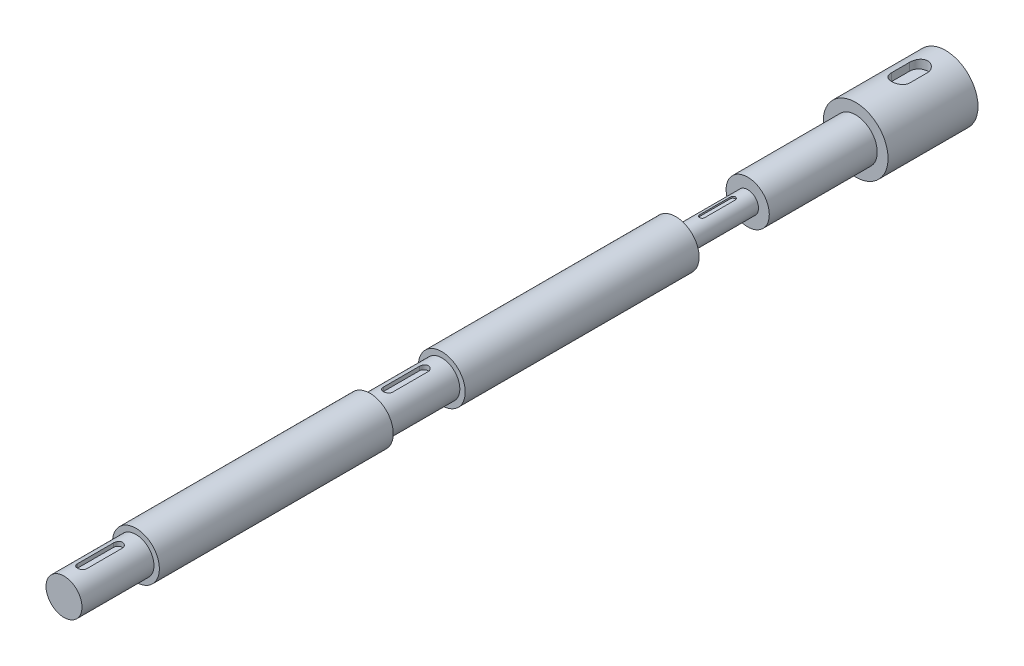
from build123d import *
from build123d.topology import SkipClean

# Parameters (mm, degrees)
SKETCH1_R           = 18
BOSS_EXTRUDE2_DEPTH = 25
SKETCH6_R           = 12
BOSS_EXTRUDE6_DEPTH = 60
SKETCH7_R           = 6
BOSS_EXTRUDE7_DEPTH = 30
CUT_EXTRUDE3_DEPTH  = 10
CUT_EXTRUDE4_DEPTH  = 5
CUT_EXTRUDE5_DEPTH  = 2.5
CUT_EXTRUDE6_DEPTH  = 2.5


with BuildPart() as part:
    # Sketch1 → Boss-Extrude2 (new, symmetric)
    with BuildSketch(Plane.XY):
        Circle(SKETCH1_R)
    extrude(amount=BOSS_EXTRUDE2_DEPTH, both=True)

    # Sketch6 → Boss-Extrude6 (add)
    with BuildSketch(Plane.XY.offset(25)):
        Circle(SKETCH6_R)
    extrude(amount=BOSS_EXTRUDE6_DEPTH)

    # Sketch7 → Boss-Extrude7 (add)
    with BuildSketch(Plane.XY.offset(85)):
        Circle(SKETCH7_R)
    extrude(amount=BOSS_EXTRUDE7_DEPTH)

    # Sketch11 → Cut-Extrude3 (cut)
    with BuildSketch(Plane(origin=(0, 13, 0), x_dir=(-1, 0, 0), z_dir=(0, 1, 0))):
        with BuildLine():
            Line((-5, 0), (-5, -10))
            ThreePointArc((-5, -10), (0, -15), (5, -10))
            Line((5, -10), (5, 0))
            ThreePointArc((5, 0), (0, 5), (-5, 0))
        make_face()
    extrude(amount=CUT_EXTRUDE3_DEPTH, mode=Mode.SUBTRACT)

    # Sketch12 → Cut-Extrude4 (cut)
    with BuildSketch(Plane(origin=(0, 5, 0), x_dir=(-1, 0, 0), z_dir=(0, 1, 0))):
        with BuildLine():
            Line((-1.4, 110.5), (-1.4, 93.3))
            ThreePointArc((-1.4, 93.3), (0, 91.9), (1.4, 93.3))
            Line((1.4, 93.3), (1.4, 110.5))
            ThreePointArc((1.4, 110.5), (0, 111.9), (-1.4, 110.5))
        make_face()
    extrude(amount=CUT_EXTRUDE4_DEPTH, mode=Mode.SUBTRACT)

    # Sketch13 → Revolve1 (revolve)
    with SkipClean():  # the faces are left unmerged after this step: merging them gives an invalid solid
        with BuildSketch(Plane(origin=(0, 0, 0), x_dir=(1, 0, 0), z_dir=(0, 1, 0))):
            Polygon((0, -465), (0, -115), (-6, -115), (-6, -125), (-13, -125), (-13, -255), (-10, -255), (-10, -295), (-13, -295), (-13, -425), (-10, -425), (-10, -465), align=None)
        revolve(axis=Axis((0, 0, 75.161405529), (0, 0, 1)))

    # Sketch16 → Cut-Extrude5 (cut)
    with SkipClean():  # the faces are left unmerged after this step: merging them gives an invalid solid
        with BuildSketch(Plane(origin=(0, 10, 0), x_dir=(1, 0, 0), z_dir=(0, 1, 0))):
            with BuildLine():
                Line((2.5, -265), (2.5, -285))
                ThreePointArc((2.5, -285), (0, -287.5), (-2.5, -285))
                Line((-2.5, -285), (-2.5, -265))
                ThreePointArc((-2.5, -265), (0, -262.5), (2.5, -265))
            make_face()
        extrude(amount=-CUT_EXTRUDE5_DEPTH, mode=Mode.SUBTRACT)

    # Sketch17 → Cut-Extrude6 (cut)
    with SkipClean():  # the faces are left unmerged after this step: merging them gives an invalid solid
        with BuildSketch(Plane(origin=(0, 10, 0), x_dir=(1, 0, 0), z_dir=(0, 1, 0))):
            with BuildLine():
                Line((2.5, -435), (2.5, -455))
                ThreePointArc((2.5, -455), (0, -457.5), (-2.5, -455))
                Line((-2.5, -455), (-2.5, -435))
                ThreePointArc((-2.5, -435), (0, -432.5), (2.5, -435))
            make_face()
        extrude(amount=-CUT_EXTRUDE6_DEPTH, mode=Mode.SUBTRACT)


solid = part.part
